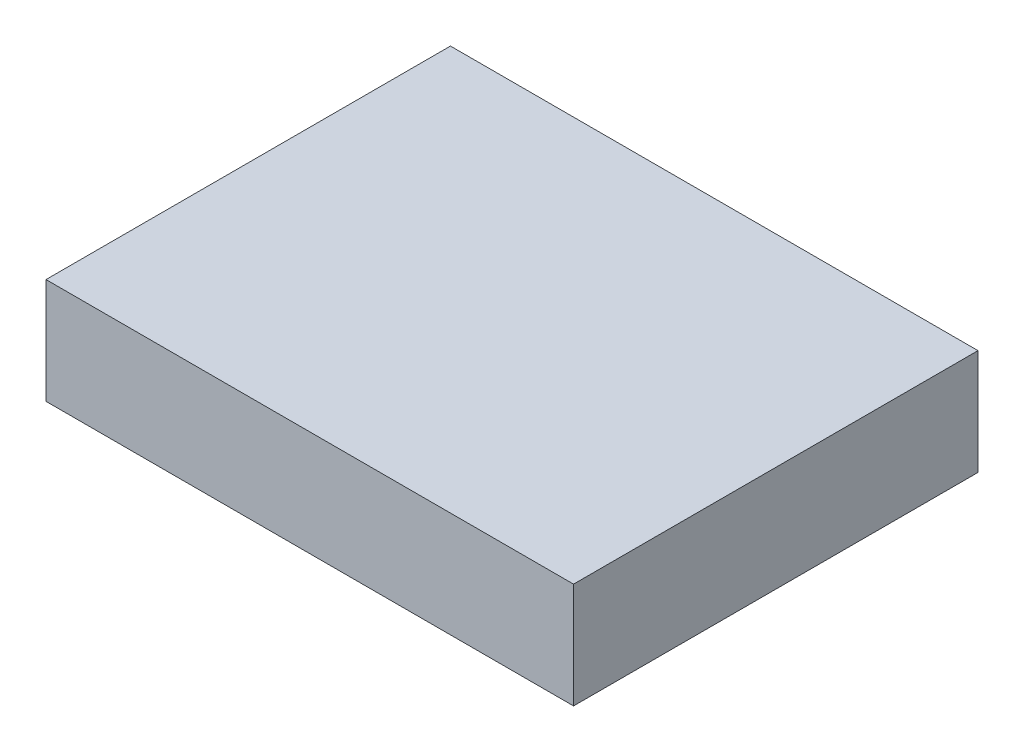
SolidWorks part; units mm, degrees
material "1023 碳钢板 (SS)"
ref_plane "Front Plane" through (0, 0, 0) normal (0, 0, 1) x (1, 0, 0)
ref_plane "Top Plane" through (0, 0, 0) normal (0, 1, 0) x (1, 0, 0)
ref_plane "Right Plane" through (0, 0, 0) normal (1, 0, 0) x (0, 0, -1)
sketch "Sketch1" plane through (0, 0, 0) normal (0, 1, 0) x (1, 0, 0)
  line L0 (30, -46) -> (30, 0) construction
  line L1 (0, 0) -> (60, 0)
  line L2 (0, 0) -> (0, -46)
  line L3 (0, -46) -> (60, -46)
  line L4 (60, 0) -> (60, -46)
  circle A0 centre (30, -21) radius 4 construction
  dimension "D3" = 8
  dimension "D1" = 60
  dimension "D2" = 46
  dimension "D4" = 25
extrude "Boss-Extrude1" add sketch "Sketch1" along normal blind 12
